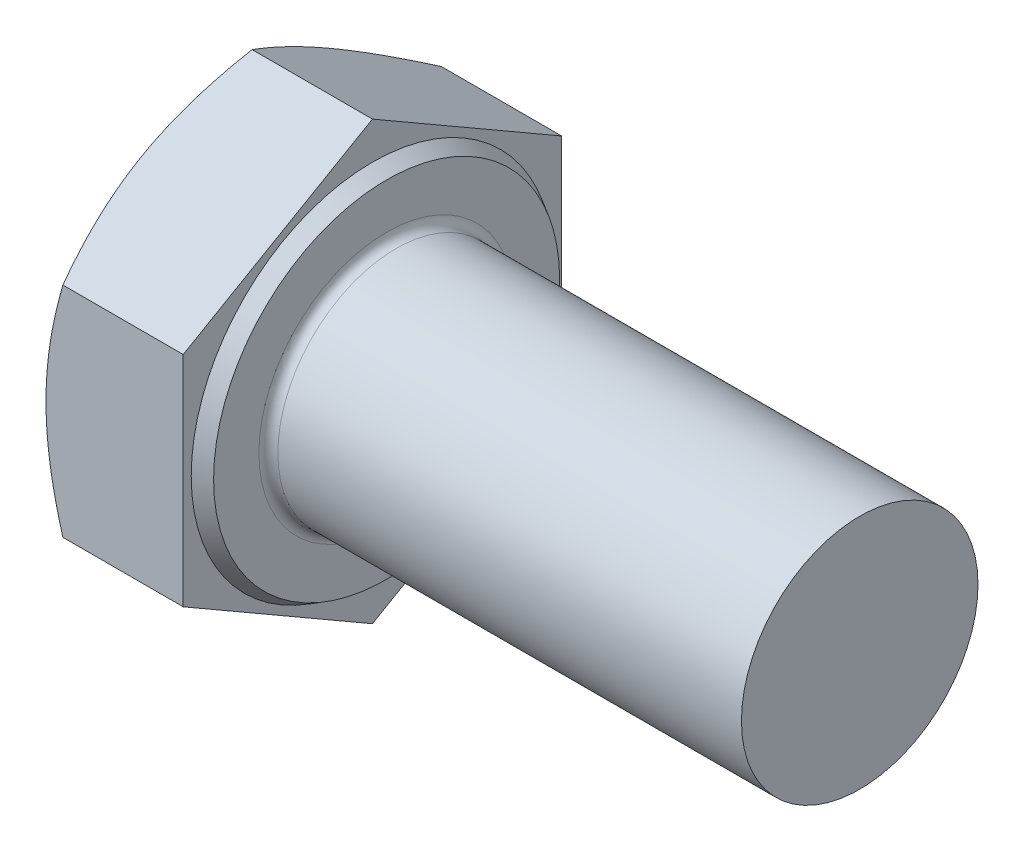
from build123d import *

# Parameters (mm, degrees)
EXTRUDE_387_DEPTH = 6.4
FILLET_1310_R     = 0.4


with BuildPart() as part:
    # 草图1 → Extrude 387 (new body)
    with BuildSketch(Plane(origin=(0, 0, 0), x_dir=(0, 0, -1), z_dir=(1, 0, 0))):
        Polygon((8, 4.618802154), (8, -4.618802154), (0, -9.237604307), (-8, -4.618802154), (-8, 4.618802154), (0, 9.237604307), align=None)
    extrude(amount=EXTRUDE_387_DEPTH)

    # 草图2 → 凸台-旋转1 (revolve)
    with BuildSketch(Plane.XY, mode=Mode.PRIVATE) as revolve_1_sk:
        Polygon((0, 0), (26.4, 0), (26.4, 3.701), (26.4, 5), (11.4, 5), (0, 5), align=None)
    revolve(revolve_1_sk.sketch.rotate(Axis((0, 0, 0), (1, 0, 0)), 90), axis=Axis((0, 0, 0), (1, 0, 0)))

    # 草图3 → 切除-旋转1 (revolve, cut)
    with BuildSketch(Plane.XY):
        Polygon((0, 8), (3.601282526, 14.237604307), (3.601282526, 19.237604307), (-10, 19.237604307), (-10, 8), align=None)
    revolve(axis=Axis((0, 0, 0), (1, 0, 0)), mode=Mode.SUBTRACT)

    # 草图4 → 切除-旋转3 (revolve, cut)
    with BuildSketch(Plane.XY, mode=Mode.PRIVATE) as cut_revolve_3_sk:
        Polygon((6.4, 7.315), (5.8, 7.661410162), (5.8, 9.237604307), (6.4, 9.237604307), align=None)
    revolve(cut_revolve_3_sk.sketch.rotate(Axis((0, 0, 0), (1, 0, 0)), 90), axis=Axis((0, 0, 0), (1, 0, 0)), mode=Mode.SUBTRACT)

    # Fillet 1310
    fillet_1310_edges = [part.edges().sort_by_distance(p)[0] for p in [
        (6.4, 0, -5),
    ]]
    fillet(fillet_1310_edges, radius=FILLET_1310_R)


solid = part.part
